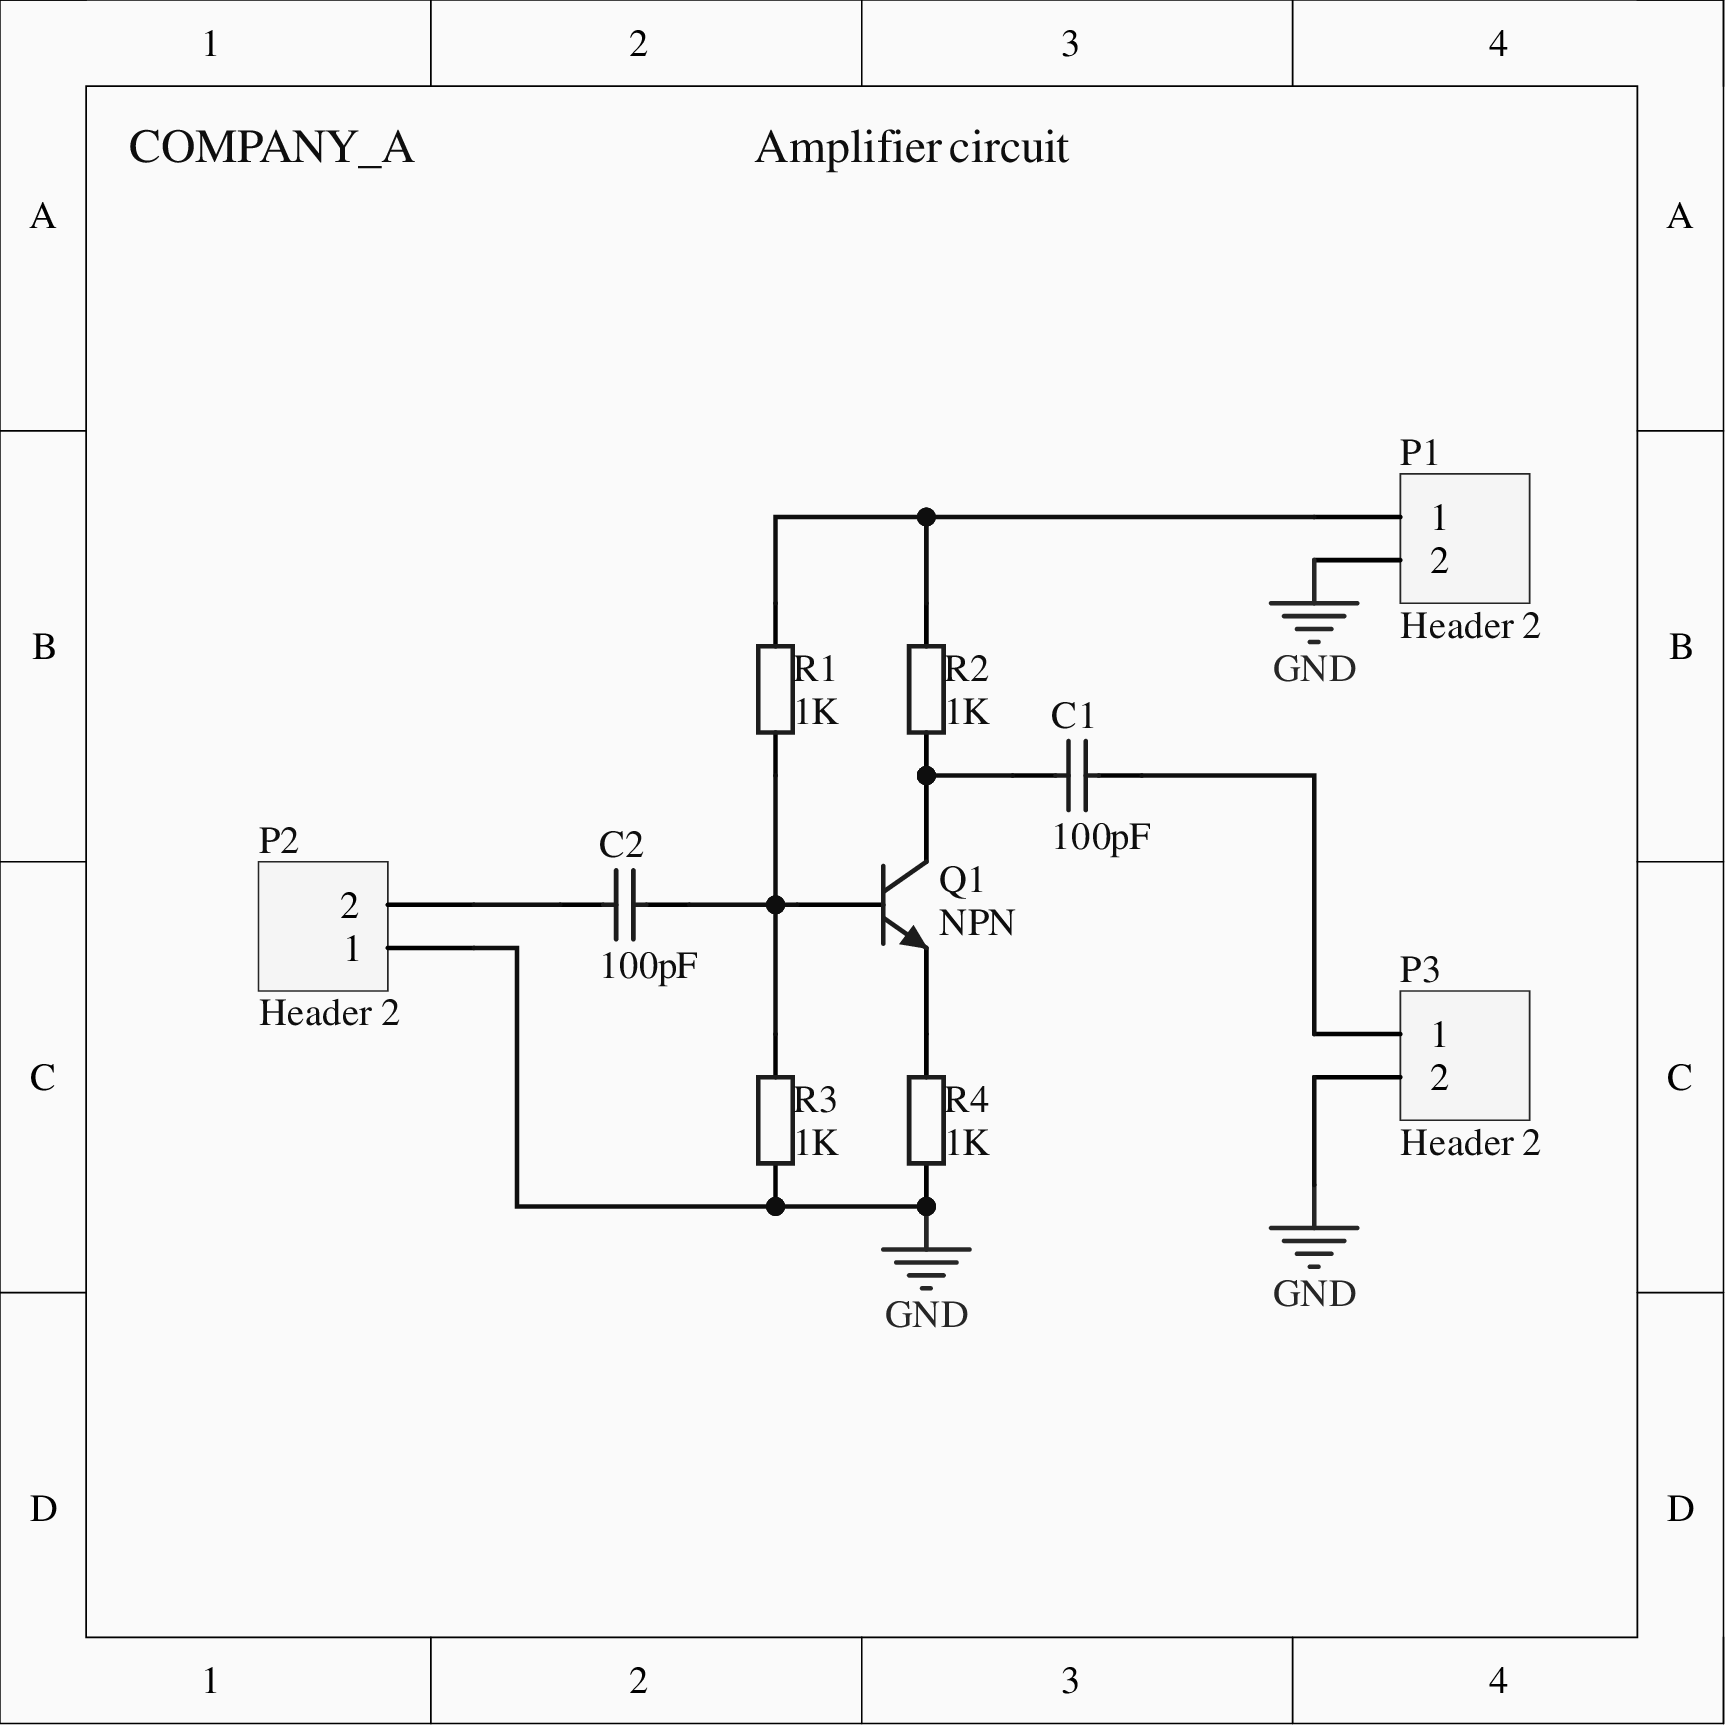
[diagram p0: MISC80548-6.SchDoc]
# Altium project MISC80548.PrjPcb
1 sheet, 10 parts. Net scope: global (net labels, ports and power ports of the same name join across sheets).
Board file: MISC80548.PcbDoc

## Sheet MISC80548-6.SchDoc
size 101 x 101 mm

### Parts
C1  100pF  [RAD-0.3]
C2  100pF  [RAD-0.3]
P1  Header 2  [HDR1X2]
P2  Header 2  [HDR1X2]
P3  Header 2  [HDR1X2]
Q1  NPN  [TO-226-AA]
R1  1K  [AXIAL-0.4]
R2  1K  [AXIAL-0.4]
R3  1K  [AXIAL-0.4]
R4  1K  [AXIAL-0.4]

### Nets
GND: P1.2 P2.1 P3.2 R3.1 R4.1
NetC1_1: C1.1 Q1.1(C) R2.1
NetC1_2: C1.2 P3.1
NetC2_1: C2.1 P2.2
NetC2_2: C2.2 Q1.2(B) R1.1 R3.2
NetP1_1: P1.1 R1.2 R2.2
NetQ1_3: Q1.3(E) R4.2

### Notes on the sheet
- COMPANY_A
- Amplifier circuit

### Library data of the parts
C1 C2 = Cap: Capacitor; Published: 8-Jun-2000; LatestRevisionDate: 17-Jul-2002; LatestRevisionNote: Re-released for DXP Platform.; PackageReference: RAD-0.3; PackageDescription: Radial Cap, Thru-Hole; 2 Leads; 0.3 in Pin Spacing; Value: 100pF; Publisher: Altium Limited
P1-P3 = Header 2: Header, 2-Pin; LatestRevisionDate: 17-Jul-2002; LatestRevisionNote: Re-released for DXP Platform.; Publisher: Altium Limited
Q1 = NPN: NPN Bipolar Transistor; Published: 8-Jun-2000; LatestRevisionDate: 17-Jul-2002; LatestRevisionNote: Re-released for DXP Platform.; PackageReference: TO-226-AA; PackageDescription: TO, Flat Index; 3 In-Line, Axial Leads; Body Dia. 4.8mm; Leads 0.55 x 0.51 mm (max); Code_JEDEC: TO-226-AA; Publisher: Altium Limited
R1-R4 = Res2: Resistor; Published: 8-Jun-2000; LatestRevisionDate: 17-Jul-2002; LatestRevisionNote: Re-released for DXP Platform.; PackageReference: AXIAL-0.4; PackageDescription: Axial Device, Thru-Hole; 2 Leads; 0.4 in Pin Spacing; Value: 1K; Publisher: Altium Limited